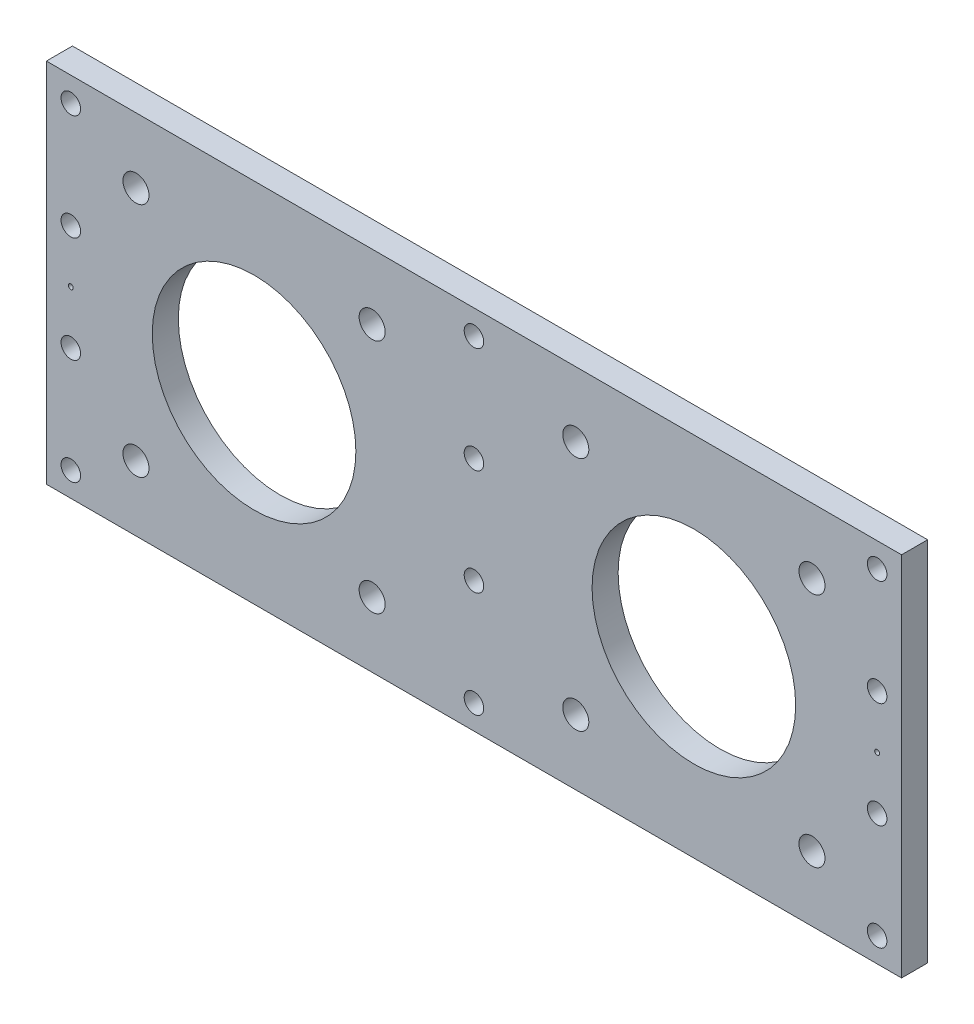
from build123d import *

# Parameters (mm, degrees)
SKETCH1_W           = 1050
SKETCH1_H           = 450
BOSS_EXTRUDE1_DEPTH = 32
SKETCH2_R           = 125
CUT_EXTRUDE1_DEPTH  = 32
SKETCH3_R           = 12
CUT_EXTRUDE2_DEPTH  = 32
SKETCH7_R           = 3
CUT_EXTRUDE3_DEPTH  = 32
CIRPATTERN1_COUNT   = 4


with BuildPart() as part:
    # Sketch1 → Boss-Extrude1 (new body)
    with BuildSketch(Plane.XY):
        with Locations((451.017205348, 170.059190469)):
            Rectangle(SKETCH1_W, SKETCH1_H)
    extrude(amount=BOSS_EXTRUDE1_DEPTH)

    # Sketch2 → Cut-Extrude1 (cut)
    with BuildSketch(Plane.XY.offset(32)):
        with Locations((181.017205348, 170.059190469)):
            Circle(SKETCH2_R)
        with Locations((721.017205348, 170.059190469)):
            Circle(SKETCH2_R)
    extrude(amount=-CUT_EXTRUDE1_DEPTH, mode=Mode.SUBTRACT)

    # Sketch3 → Cut-Extrude2 (cut)
    with BuildSketch(Plane.XY.offset(32)):
        with Locations((-43.982794652, 365.059190469)):
            Circle(SKETCH3_R)
        with Locations((-43.982794652, 235.059190469)):
            Circle(SKETCH3_R)
        with Locations((-43.982794652, 105.059190469)):
            Circle(SKETCH3_R)
        with Locations((-43.982794652, -24.940809531)):
            Circle(SKETCH3_R)
        with Locations(Location((946.017205348, -24.940809531, 0), (0, 0, 180))):
            Circle(SKETCH3_R)
        with Locations(Location((946.017205348, 105.059190469, 0), (0, 0, 180))):
            Circle(SKETCH3_R)
        with Locations(Location((946.017205348, 235.059190469, 0), (0, 0, 180))):
            Circle(SKETCH3_R)
        with Locations(Location((946.017205348, 365.059190469, 0), (0, 0, 180))):
            Circle(SKETCH3_R)
        with Locations((451.017205348, 365.059190469)):
            Circle(SKETCH3_R)
        with Locations((451.017205348, 235.059190469)):
            Circle(SKETCH3_R)
        with Locations((451.017205348, 105.059190469)):
            Circle(SKETCH3_R)
        with Locations((451.017205348, -24.940809531)):
            Circle(SKETCH3_R)
    extrude(amount=-CUT_EXTRUDE2_DEPTH, mode=Mode.SUBTRACT)

    # Sketch5 → M36 Tapped Hole1 (revolve, cut)
    with BuildSketch(Plane(origin=(36.017205348, 315.059190469, 32), x_dir=(0, -1, 0), z_dir=(1, 0, 0))):
        Polygon((0, 0), (0, 101.613769904), (16, 92), (16, 0), align=None)
    m36_tapped_hole1 = revolve(axis=Axis((36.017205348, 315.059190469, 38.35), (0, 0, -1)), mode=Mode.SUBTRACT)

    # Mirror1: M36 Tapped Hole1 across plane
    add(m36_tapped_hole1.mirror(Plane.ZY.offset(-451.017205348)), mode=Mode.SUBTRACT)

    # Sketch7 → Cut-Extrude3 (cut)
    with BuildSketch(Plane.XY.offset(32)):
        with Locations((-43.982794652, 170.059190469)):
            Circle(SKETCH7_R)
    cut_extrude3 = extrude(amount=-CUT_EXTRUDE3_DEPTH, mode=Mode.SUBTRACT)

    # Mirror2: Cut-Extrude3 across plane
    add(cut_extrude3.mirror(Plane.ZY.offset(-451.017205348)), mode=Mode.SUBTRACT)

    # CirPattern1: M36 Tapped Hole1 ×4 about axis
    cirpattern1_axis = Axis((181.017205348, 170.059190469, 0), (0, 0, 1))
    for i in range(1, CIRPATTERN1_COUNT):
        add(m36_tapped_hole1.rotate(cirpattern1_axis, i * 360 / CIRPATTERN1_COUNT), mode=Mode.SUBTRACT)

    # Mirror3: M36 Tapped Hole1 across plane
    add(m36_tapped_hole1.mirror(Plane.ZY.offset(-451.017205348)), mode=Mode.SUBTRACT)

    # Mirror3 copy 1 sketch → Mirror3 copy 1 (revolve, cut)
    with BuildSketch(Plane(origin=(866.017205348, 25.059190469, 32), x_dir=(-1, 0, 0), z_dir=(0, 1, 0))):
        Polygon((0, 0), (0, -101.613769904), (16, -92), (16, 0), align=None)
    revolve(axis=Axis((866.017205348, 25.059190469, 38.35), (0, 0, 1)), mode=Mode.SUBTRACT)

    # Mirror3 copy 2 sketch → Mirror3 copy 2 (revolve, cut)
    with BuildSketch(Plane(origin=(576.017205348, 25.059190469, 32), x_dir=(0, 1, 0), z_dir=(1, 0, 0))):
        Polygon((0, 0), (0, -101.613769904), (16, -92), (16, 0), align=None)
    revolve(axis=Axis((576.017205348, 25.059190469, 38.35), (0, 0, 1)), mode=Mode.SUBTRACT)

    # Mirror3 copy 3 sketch → Mirror3 copy 3 (revolve, cut)
    with BuildSketch(Plane(origin=(576.017205348, 315.059190469, 32), x_dir=(1, 0, 0), z_dir=(0, -1, 0))):
        Polygon((0, 0), (0, -101.613769904), (16, -92), (16, 0), align=None)
    revolve(axis=Axis((576.017205348, 315.059190469, 38.35), (0, 0, 1)), mode=Mode.SUBTRACT)


solid = part.part
